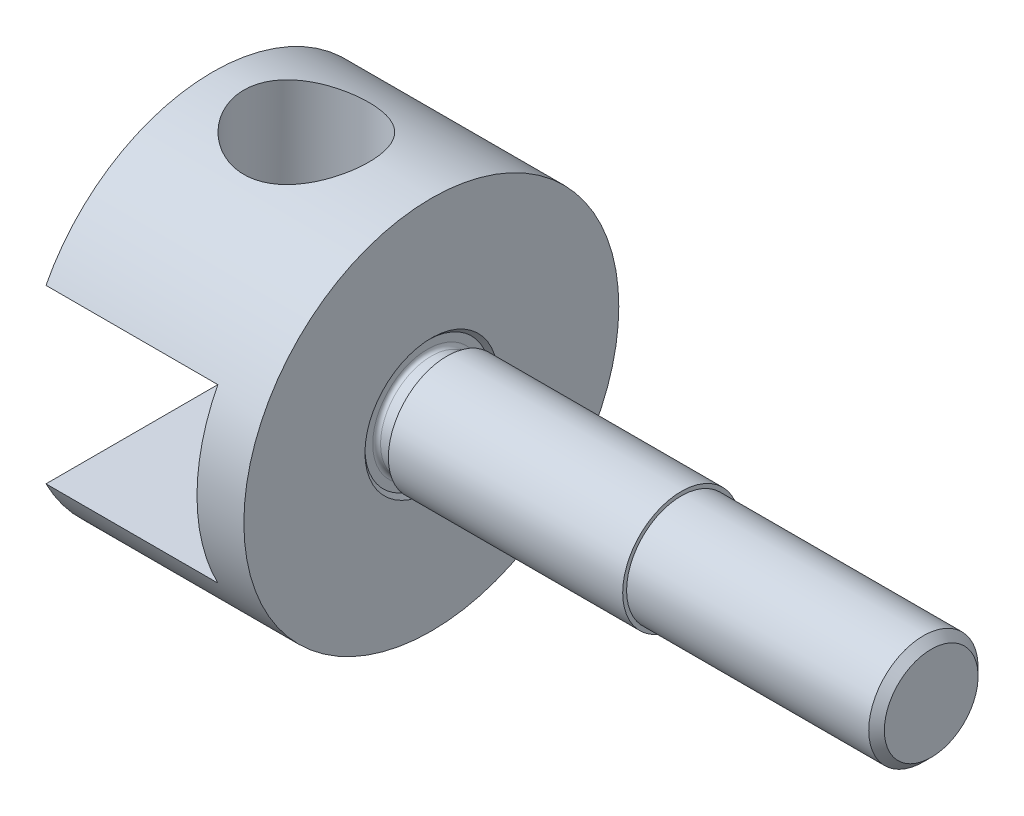
SolidWorks part; units mm, degrees
ref_plane "Front Plane" through (0, 0, 0) normal (0, 0, 1) x (1, 0, 0)
ref_plane "Top Plane" through (0, 0, 0) normal (0, 1, 0) x (1, 0, 0)
ref_plane "Right Plane" through (0, 0, 0) normal (1, 0, 0) x (0, 0, -1)
other "Configuration Table"
sketch "Sketch1" plane through (0, 0, 0) normal (0, 0, 1) x (1, 0, 0)
  line L0 (-36.1818, 0) -> (50.5455, 0) construction
  line L1 (0, 0) -> (0, 24)
  line L2 (0, 24) -> (28, 24)
  line L3 (28, 24) -> (28, 7)
  line L4 (28, 7) -> (30, 7)
  line L5 (30, 7) -> (30, 7.5)
  line L6 (30, 7.5) -> (60, 7.5)
  line L7 (60, 7.5) -> (60, 7)
  line L8 (60, 7) -> (92, 7)
  line L9 (92, 7) -> (92, 0)
  line L10 (92, 0) -> (0, 0)
  dimension "D1" = 28
  dimension "D2" = 24
  dimension "D3" = 32
  dimension "D4" = 92
  dimension "D5" = 7
  dimension "D6" = 7.5
  dimension "D7" = 7
  dimension "D8" = 2
revolve "Revolve1" add sketch "Sketch1" angle 360 about L0
sketch "Sketch2" plane through (0, 0, 0) normal (-1, 0, 0) x (0, 0, 1)
  line L1 (42.399, -11) -> (-42.399, -11)
  line L2 (42.399, -11) -> (42.399, 11)
  line L3 (42.399, 11) -> (-42.399, 11)
  line L4 (-42.399, -11) -> (-42.399, 11)
  line L5 (42.399, -11) -> (-42.399, 11) construction
  line L6 (42.399, 11) -> (-42.399, -11) construction
  point P0 (0, 0)
  dimension "D1" = 22
extrude "Cut-Extrude1" cut sketch "Sketch2" against normal blind 22
sketch "Sketch3" plane through (0, -11, 0) normal (0, 1, 0) x (1, 0, 0)
  line L0 (0, 21.3307) -> (0, -21.3307) construction
  circle A0 centre (12, 0) radius 8
  dimension "D2" = 16
  dimension "D1" = 12
extrude "Cut-Extrude2" cut sketch "Sketch3" against normal blind 22 and the other way blind 51
sketch "Sketch7" plane through (0, 0, 0) normal (0, 1, 0) x (1, 0, 0)
  line L1 (27.5, -7) -> (27.5, -8)
  line L2 (27.5, -8) -> (28, -8.5)
  line L3 (28, -8.5) -> (28, -7)
  line L4 (28, -7) -> (30, -7)
  line L5 (28, -24) -> (28, 24) construction
  line L6 (28, -6.5) -> (29.5, -6.5)
  line L7 (29.5, -6.5) -> (30, -7)
  line L8 (28, -7) -> (30, -7) construction
  line L9 (0, 0) -> (67.04, 0) construction
  arc A0 (28, -6.5) -> (27.5, -7) centre (28, -7) ccw
  dimension "D2" = 1.5
  dimension "D1" = 0.5
  dimension "D3" = 45
  dimension "D4" = 45
  dimension "D5" = 2
  dimension "D6" = 0.5
revolve "Cut-Revolve1" cut sketch "Sketch7" angle 360 about L9
chamfer "Chamfer1" distance 1 angle 45 1 edges at (92, 0, 7)
